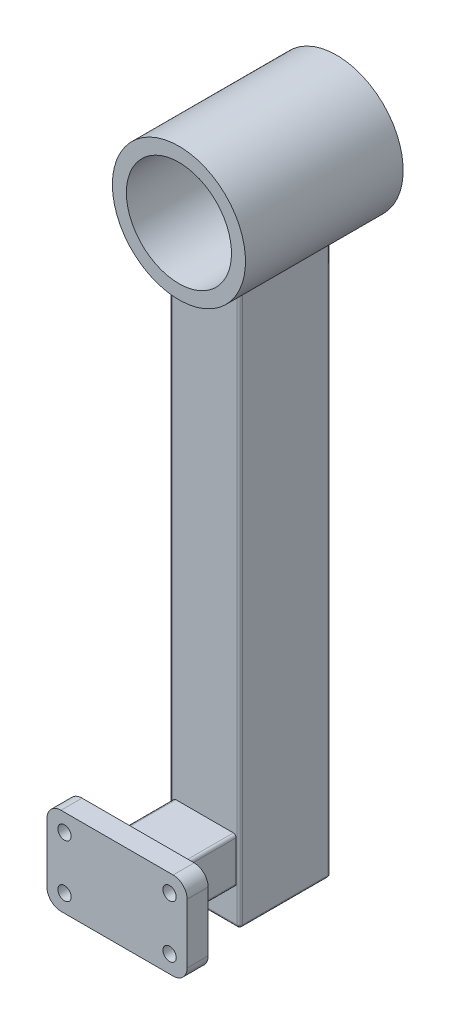
from build123d import *

# Parameters (mm, degrees)
SKETCH1_R                = 1.9
BOSS_EXTRUDE1_DEPTH      = 6
SKETCH2_W                = 18
SKETCH2_H                = 13
BOSS_EXTRUDE2_DEPTH      = 32
BOSS_EXTRUDE3_DEPTH      = 10
BOSS_EXTRUDE3_DEPTH_BACK = 150
SKETCH4_W                = 20
SKETCH4_H                = 26
BOSS_EXTRUDE4_DEPTH      = 10
BOSS_EXTRUDE4_DEPTH_BACK = 35
SKETCH5_R                = 19
SKETCH5_R_2              = 15
FILLET1_R                = 0.8


with BuildPart() as part:
    # Sketch1 → Boss-Extrude1 (new body)
    with BuildSketch(Plane.XY):
        with BuildLine():
            Line((-16, 12.5), (16, 12.5))
            ThreePointArc((16, 12.5), (18.828427125, 11.328427125), (20, 8.5))
            Line((20, 8.5), (20, -8.5))
            ThreePointArc((20, -8.5), (18.828427125, -11.328427125), (16, -12.5))
            Line((16, -12.5), (-16, -12.5))
            ThreePointArc((-16, -12.5), (-18.828427125, -11.328427125), (-20, -8.5))
            Line((-20, -8.5), (-20, 8.5))
            ThreePointArc((-20, 8.5), (-18.828427125, 11.328427125), (-16, 12.5))
        make_face()
        with Locations((-15, 7.5)):
            Circle(SKETCH1_R, mode=Mode.SUBTRACT)
        with Locations((15, 7.5)):
            Circle(SKETCH1_R, mode=Mode.SUBTRACT)
        with Locations((15, -7.5)):
            Circle(SKETCH1_R, mode=Mode.SUBTRACT)
        with Locations((-15, -7.5)):
            Circle(SKETCH1_R, mode=Mode.SUBTRACT)
    extrude(amount=BOSS_EXTRUDE1_DEPTH)

    # Sketch2 → Boss-Extrude2 (add)
    with BuildSketch(Plane(origin=(0, 0, 0), x_dir=(-1, 0, 0), z_dir=(0, 0, -1))):
        Rectangle(SKETCH2_W, SKETCH2_H)
    extrude(amount=BOSS_EXTRUDE2_DEPTH)

    # Sketch4 → Boss-Extrude3 (add, two sides: drawn at the far end of the back side and taken through both)
    with BuildSketch(Plane(origin=(0, -6.5, 0), x_dir=(-1, 0, 0), z_dir=(0, -1, 0)).offset(-BOSS_EXTRUDE3_DEPTH_BACK)):
        with Locations((0, 32)):
            Rectangle(SKETCH4_W, SKETCH4_H)
    extrude(amount=BOSS_EXTRUDE3_DEPTH + BOSS_EXTRUDE3_DEPTH_BACK)

    # Sketch5 → Boss-Extrude4 (add, two sides: drawn at the far end of the back side and taken through both)
    with BuildSketch(Plane(origin=(0, 0, -45), x_dir=(-1, 0, 0), z_dir=(0, 0, -1)).offset(-BOSS_EXTRUDE4_DEPTH_BACK)):
        with Locations((-1.66190379, 158.5)):
            Circle(SKETCH5_R)
        with Locations((-1.66190379, 158.5)):
            Circle(SKETCH5_R_2, mode=Mode.SUBTRACT)
    extrude(amount=BOSS_EXTRUDE4_DEPTH + BOSS_EXTRUDE4_DEPTH_BACK)

    # Fillet1
    fillet1_edges = [part.edges().sort_by_distance(p)[0] for p in [
        (-9, -6.5, -9.5),
        (9, -6.5, -9.5),
        (9, 6.5, -9.5),
        (-9, 6.5, -9.5),
        (-10, 63.5, -19),
        (-10, 63.5, -45),
        (10, -16.5, -32),
        (0, -16.5, -19),
        (-10, -16.5, -32),
        (0, -16.5, -45),
        (10, 62.463663672, -45),
        (10, 62.463663672, -19),
    ]]
    fillet(fillet1_edges, radius=FILLET1_R)


solid = part.part
